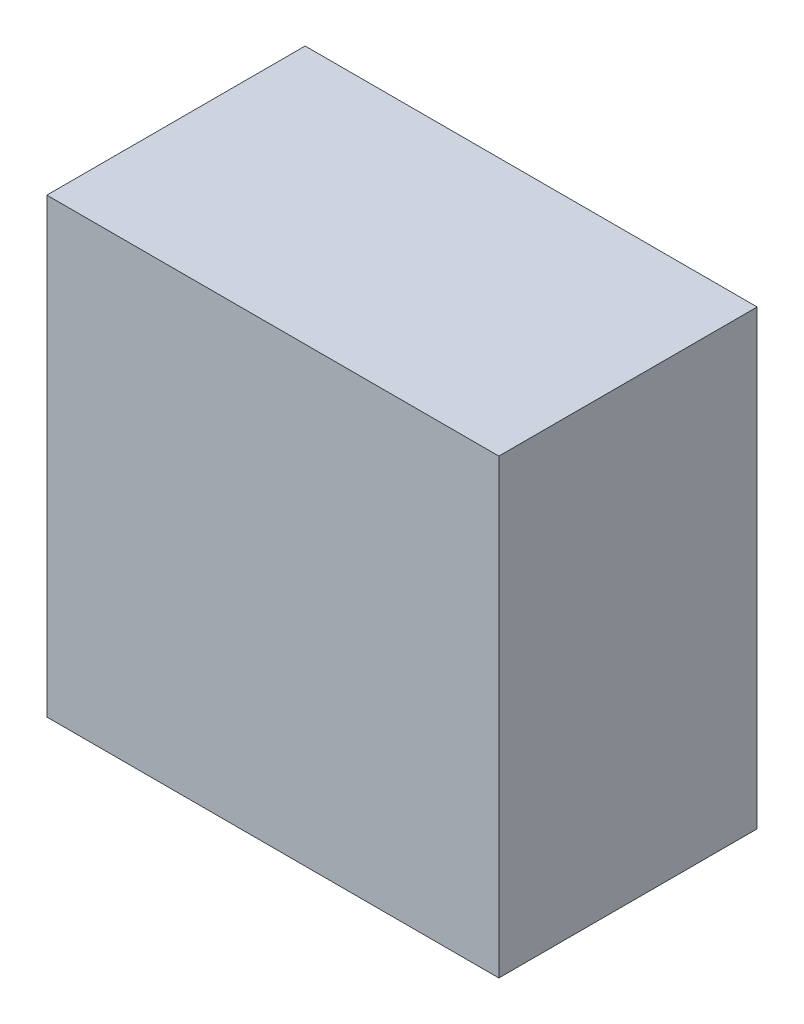
from build123d import *

# Parameters (mm, degrees)
SKETCH1_W           = 35
SKETCH1_H           = 35
BOSS_EXTRUDE1_DEPTH = 20
SHELL1_T            = -1


with BuildPart() as part:
    # Sketch1 → Boss-Extrude1 (new body)
    with BuildSketch(Plane.XY):
        with Locations((-91.5, -21.5)):
            Rectangle(SKETCH1_W, SKETCH1_H)
    extrude(amount=-BOSS_EXTRUDE1_DEPTH)

    # Shell1
    shell1_openings = [part.faces().sort_by_distance(p)[0] for p in [
        (-91.5, -21.5, -20),
    ]]
    offset(amount=SHELL1_T, openings=shell1_openings, kind=Kind.INTERSECTION)


solid = part.part
